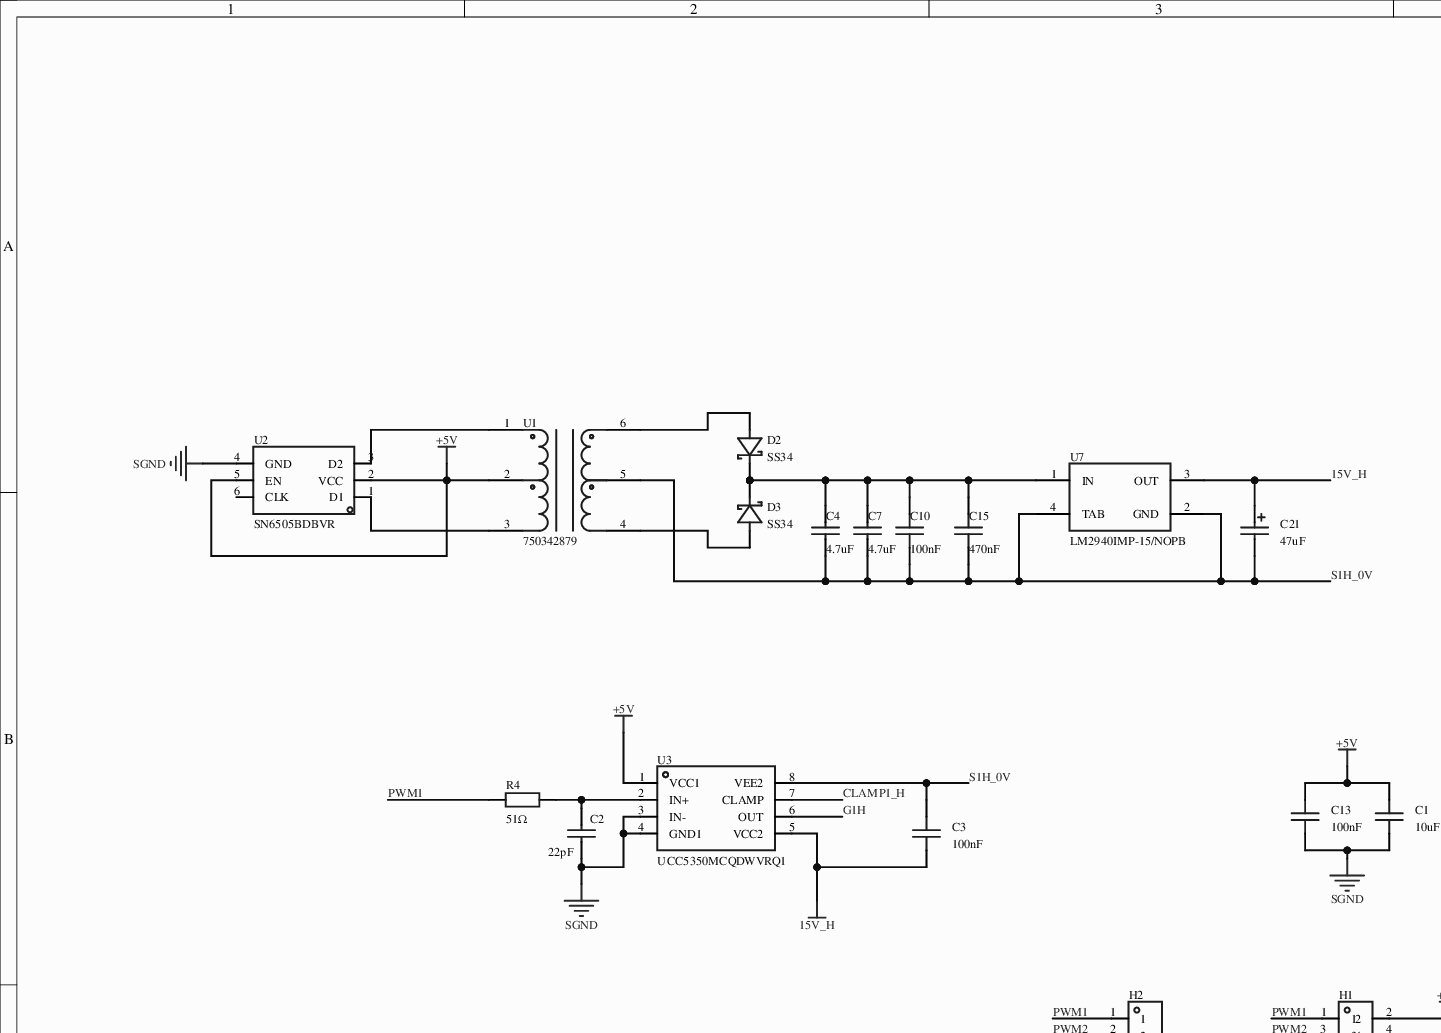
[diagram p0: MISC51425-3.schdoc, top left]
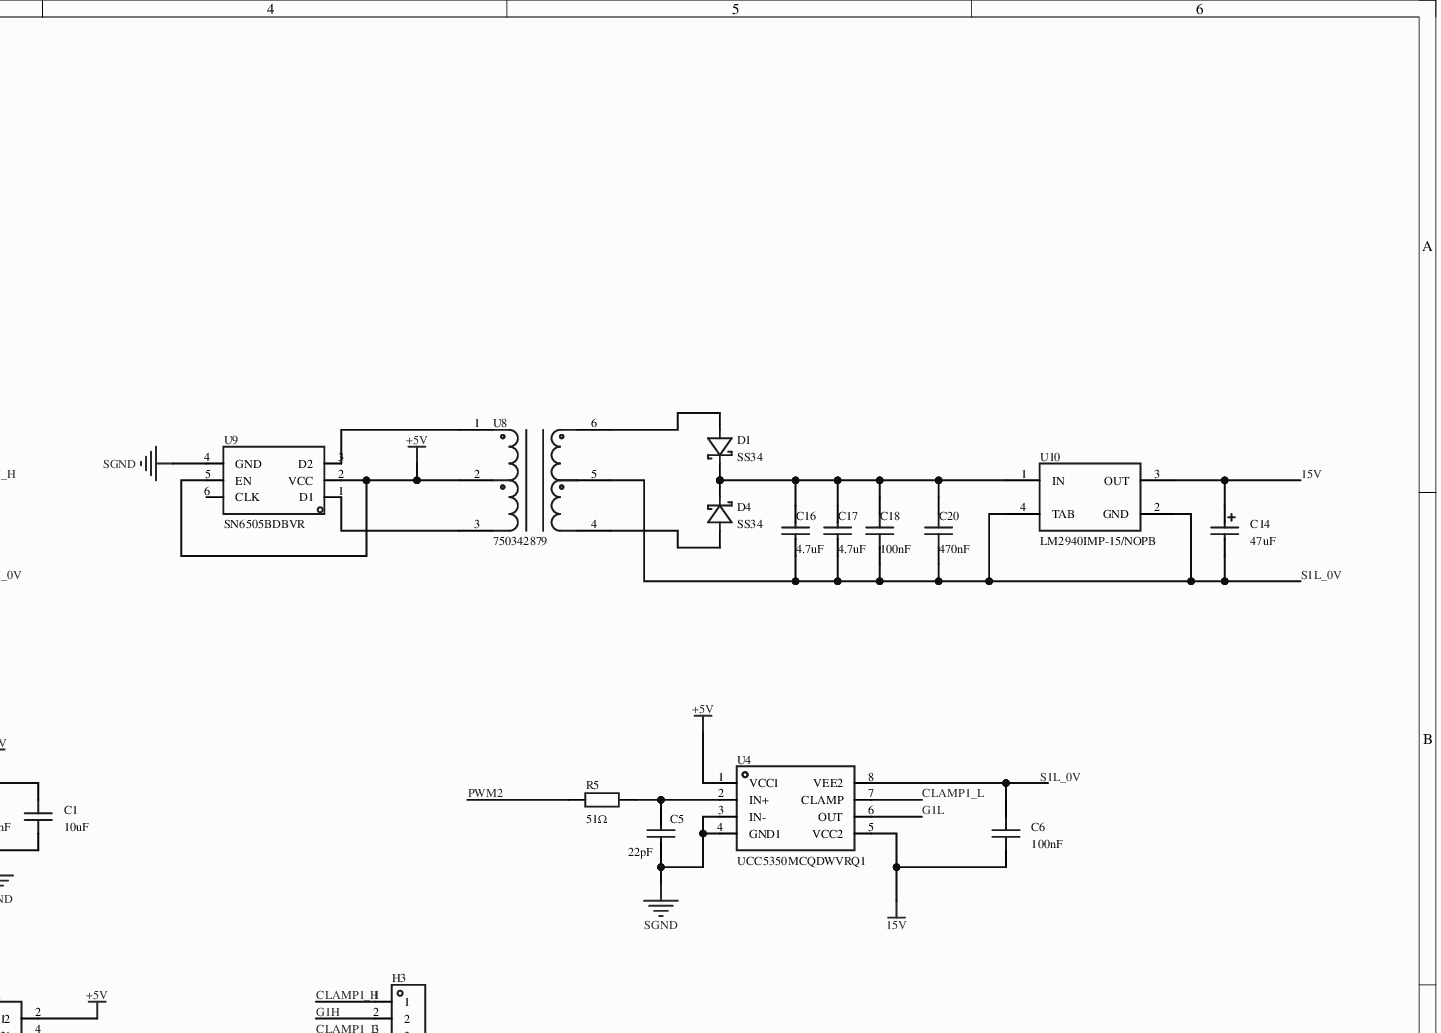
[diagram p1: MISC51425-3.schdoc, top right]
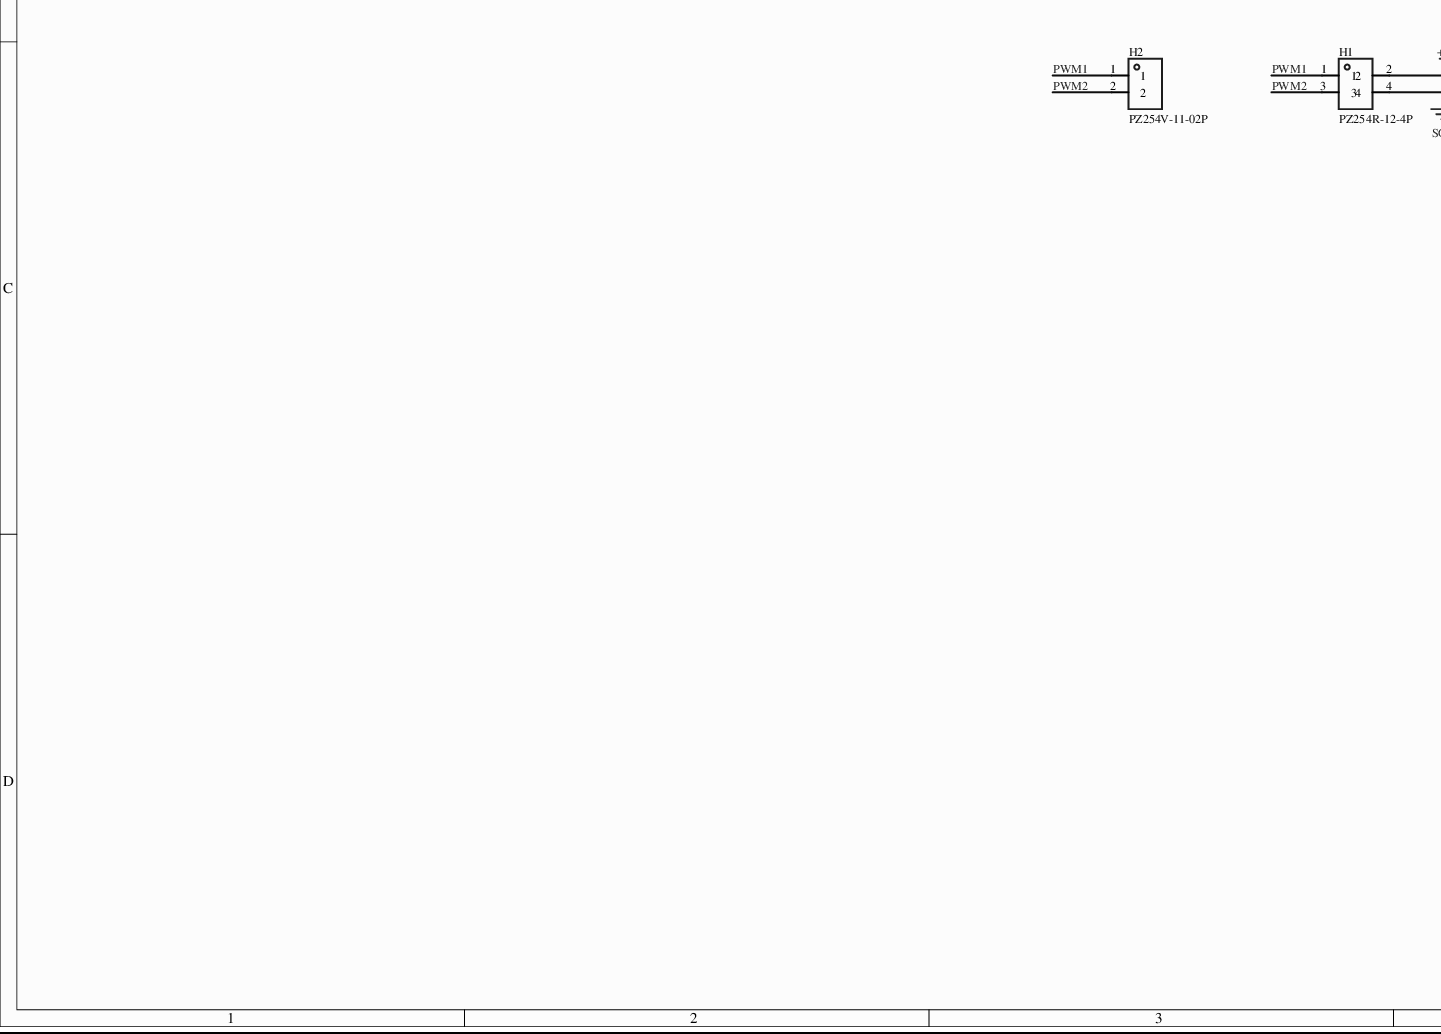
[diagram p2: MISC51425-3.schdoc, bottom left]
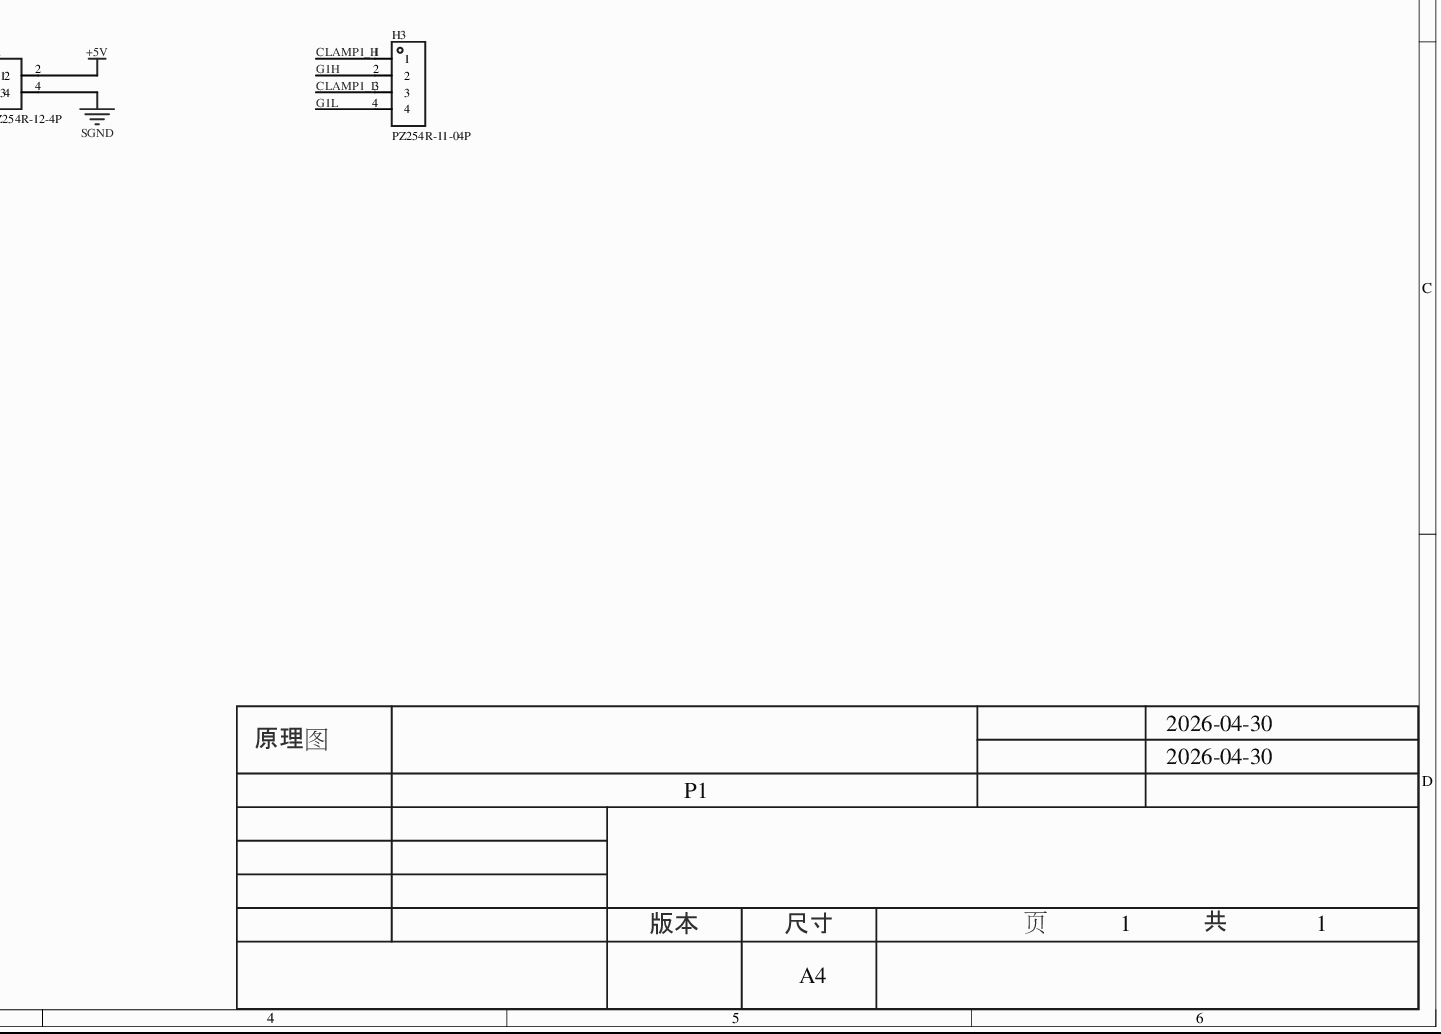
[diagram p3: MISC51425-3.schdoc, bottom right]
# Altium project MISC51425-2.PrjPcb
1 sheet, 33 parts. Net scope: global (net labels, ports and power ports of the same name join across sheets).
Board file: MISC51425.pcbdoc

## Sheet MISC51425-3.schdoc
size 420 x 297 mm; Version: V1.0; @Project Name: MISC51425; @Page Count: 1; @Update Date: 2026-04-30; @Create Date: 2026-04-30; @Schematic Name: MISC51425; @Page No: 1; @Board Name: MISC51425; @Update Time: 15:18:57; @Create Time: 15:18:57

### Parts
C1  10uF  [C0603]
C2  22pF  [C0402]
C3  100nF  [C0603]
C4  4.7uF  [C0805]
C5  22pF  [C0402]
C6  100nF  [C0603]
C7  4.7uF  [C0805]
C10  100nF  [CAP-SMD_L2.0-W1.25]
C13  100nF  [C0603]
C14  47uF  [CAP-SMD_L7.3-W4.3-FD]
C15  470nF  [C0603]
C16  4.7uF  [C0805]
C17  4.7uF  [C0805]
C18  100nF  [CAP-SMD_L2.0-W1.25]
C20  470nF  [C0603]
C21  47uF  [CAP-SMD_L7.3-W4.3-FD]
D1  SS34  [SMA_L4.3-W2.6-LS5.0-FD]
D2  SS34  [SMA_L4.3-W2.6-LS5.0-FD]
D3  SS34  [SMA_L4.3-W2.6-LS5.0-FD]
D4  SS34  [SMA_L4.3-W2.6-LS5.0-FD]
H1  PZ254R-12-4P  [HDR-TH_4P-P2.54-H-M-R2-C2-S2.54]
H2  PZ254V-11-02P  [HDR-TH_2P-P2.54-V-M]
H3  PZ254R-11-04P  [HDR-TH_4P-P2.54-H-M-W10.4]
R4  51Ω  [R0603]
R5  51Ω  [R0603]
U1  750342879  [XFMR-SMD_6P-L9.1-W8.0-P3.05-LS13.0-TL]
U2  SN6505BDBVR  [SOT-23-6_L2.9-W1.6-P0.95-LS2.8-BR]
U3  UCC5350MCQDWVRQ1  [SOIC-8_L7.5-W5.9-P1.27-LS11.5-BL]
U4  UCC5350MCQDWVRQ1  [SOIC-8_L7.5-W5.9-P1.27-LS11.5-BL]
U7  LM2940IMP-15/NOPB  [SOT-223-3_L6.5-W3.4-P2.30-LS7.0-BR]
U8  750342879  [XFMR-SMD_6P-L9.1-W8.0-P3.05-LS13.0-TL]
U9  SN6505BDBVR  [SOT-23-6_L2.9-W1.6-P0.95-LS2.8-BR]
U10  LM2940IMP-15/NOPB  [SOT-223-3_L6.5-W3.4-P2.30-LS7.0-BR]

### Nets
15V: C6.2 C14.1 U4.5(VCC2) U10.3(OUT)
15V_H: C3.2 C21.1 U3.5(VCC2) U7.3(OUT)
+5V: C1.1 C13.1 H1.2 U1.2 U2.2(VCC) U2.5(EN) U3.1(VCC1) U4.1(VCC1) U8.2 U9.2(VCC) U9.5(EN)
SGND: C1.2 C2.1 C5.1 C13.2 H1.4 U2.4(GND) U3.3(IN-) U3.4(GND1) U4.3(IN-) U4.4(GND1) U9.4(GND)
CLAMP1_H: H3.1 U3.7(CLAMP)
CLAMP1_L: H3.3 U4.7(CLAMP)
G1H: H3.2 U3.6(OUT)
G1L: H3.4 U4.6(OUT)
PWM1: H1.1 H2.1 R4.1
PWM2: H1.3 H2.2 R5.1
S1H_0V: C3.1 C4.1 C7.1 C10.1 C15.1 C21.2 U1.5 U3.8(VEE2) U7.2(GND) U7.4(TAB)
S1L_0V: C6.1 C14.2 C16.1 C17.1 C18.1 C20.1 U4.8(VEE2) U8.5 U10.2(GND) U10.4(TAB)
NetC2_2: C2.2 R4.2 U3.2(IN+)
NetC4_2: C4.2 C7.2 C10.2 C15.2 D2.2(K) D3.2(K) U7.1(IN)
NetC5_2: C5.2 R5.2 U4.2(IN+)
NetC16_2: C16.2 C17.2 C18.2 C20.2 D1.2(K) D4.2(K) U10.1(IN)
NetD1_1: D1.1(A) U8.6
NetD2_1: D2.1(A) U1.6
NetD3_1: D3.1(A) U1.4
NetD4_1: D4.1(A) U8.4
NetU1_1: U1.1 U2.3(D2)
NetU1_3: U1.3 U2.1(D1)
NetU8_1: U8.1 U9.3(D2)
NetU8_3: U8.3 U9.1(D1)

Not connected (* = marked no-connect by the designer): U2 6(CLK)*; U9 6(CLK)*

### Notes on the sheet
- 2026-04-30
- 原理图
- P1
- 版本
- 尺寸
- A4
- 页
- 1
- 共

### Library data of the parts
C1 = GRM188R61E106KA73D: 容值:10uF;精度:±10%;额定电压:25V;温度系数:X5R;; Manufacturer: muRata(村田); 3D Model: ac125912035d415993ca9572d50418b10819f05c4eef4c71ace90d822a990e87; 3D Model Transform: 62.992,31.496,0,0,0,0,0,0,0; Tolerance: ±10%; Voltage Rating: 25V; Temperature Coefficient: X5R; AddInBom: yes; ModelName: C0603_L1.6-W0.8-H0.8; Device: GRM188R61E106KA73D; Symbol: GRM188R61E106KA73D; LCSC Part Name: 10uF ±10% 25V; Supplier Part: C344022; Manufacturer Part: GRM188R61E106KA73D; Supplier Footprint: 0603; JLCPCB Part Class: Extended Part; Datasheet: https://item.szlcsc.com/datasheet/GRM188R61E106KA73D/320824.html; Supplier: LCSC; Value: 10uF; FootprintName: C0603; ConvertToPcb: yes
C2 C5 = 0402CG220J500NT: 容值:22pF;精度:±5%;额定电压:50V;温度系数:C0G;; Manufacturer: FH(风华); 3D Model: 36a51122f27c49738f86b3bfa98863e00819f05c4eef4c71ace90d822a990e87; 3D Model Transform: 39.37,19.685,0,0,0,0,0,0,0; Tolerance: ±5%; Voltage Rating: 50V; Temperature Coefficient: C0G; AddInBom: yes; ModelName: C0402_L1.0-W0.5-H0.5; Device: 0402CG220J500NT; Symbol: 0402CG220J500NT; LCSC Part Name: 22pF ±5% 50V; Supplier Part: C1555; Manufacturer Part: 0402CG220J500NT; Supplier Footprint: 0402; JLCPCB Part Class: Basic Part; Datasheet: https://item.szlcsc.com/datasheet/0402CG220J500NT/1907.html; Supplier: LCSC; Value: 22pF; FootprintName: C0402; ConvertToPcb: yes
C3 C6 C13 = CGA0603X7R104K500JT: 容值:100nF;精度:±10%;额定电压:50V;温度系数:X7R;; Manufacturer: HRE(芯声); 3D Model: ac125912035d415993ca9572d50418b10819f05c4eef4c71ace90d822a990e87; 3D Model Transform: 62.992,31.496,0,0,0,0,0,0,0; Tolerance: ±10%; Voltage Rating: 50V; Temperature Coefficient: X7R; AddInBom: yes; ModelName: C0603_L1.6-W0.8-H0.8; Device: CGA0603X7R104K500JT; Symbol: CGA0603X7R104K500JT; LCSC Part Name: 100nF ±10% 50V; Supplier Part: C6119867; Manufacturer Part: CGA0603X7R104K500JT; Supplier Footprint: 0603; JLCPCB Part Class: Extended Part; Datasheet: https://item.szlcsc.com/datasheet/CGA0603X7R104K500JT/7062573.html; Supplier: LCSC; Value: 100nF; FootprintName: C0603; ConvertToPcb: yes
C4 C7 C16 C17 = CL21A475KBQNNNE: 容值:4.7uF;精度:±10%;额定电压:50V;温度系数:X5R;; Manufacturer: SAMSUNG(三星); 3D Model: 1ba041120af144c991958decab20d2410819f05c4eef4c71ace90d822a990e87; 3D Model Transform: 78.74,51.181,0,0,0,0,0,0.0005,0; Tolerance: ±10%; Voltage Rating: 50V; Temperature Coefficient: X5R; AddInBom: yes; ModelName: C0805_L2.0-W1.3-H1.3; Device: CL21A475KBQNNNE; Symbol: CL21A475KBQNNNE; LCSC Part Name: 4.7uF ±10% 50V; Supplier Part: C98192; Manufacturer Part: CL21A475KBQNNNE; Supplier Footprint: 0805; JLCPCB Part Class: Extended Part; Datasheet: https://item.szlcsc.com/datasheet/CL21A475KBQNNNE/99401.html; Supplier: LCSC; Value: 4.7uF; FootprintName: C0805; ConvertToPcb: yes
C10 C18 = FCC0805B104K500DT: 容值:100nF;精度:±10%;额定电压:50V;温度系数:X7R;; Manufacturer: FOJAN(富捷); 3D Model: dce19e309e9b4209af79576cb8c62f2f0819f05c4eef4c71ace90d822a990e87; 3D Model Transform: 78.74,49.2125,0,0,0,0,0,0,0; Tolerance: ±10%; Voltage Rating: 50V; Temperature Coefficient: X7R; AddInBom: yes; ModelName: CAP-SMD_L2.0-W1.3-H1.3; Device: FCC0805B104K500DT; Symbol: FCC0805B104K500DT; LCSC Part Name: 100nF ±10% 50V; Supplier Part: C5137467; Manufacturer Part: FCC0805B104K500DT; Supplier Footprint: 0805; JLCPCB Part Class: Extended Part; Datasheet: https://item.szlcsc.com/datasheet/FCC0805B104K500DT/5746969.html; Supplier: LCSC; Value: 100nF; FootprintName: CAP-SMD_L2.0-W1.25; ConvertToPcb: yes
C14 C21 = T491X476K035AT: 容值:47uF;精度:±10%;额定电压:35V;等效串联电阻(ESR):600mΩ@100kHz;; Manufacturer: KEMET(基美); 3D Model: a7253e4667014c2b8171994ff34e6c410819f05c4eef4c71ace90d822a990e87; 3D Model Transform: 287.402,169.291,0,0,0,0,-0.1,0,0; Tolerance: ±10%; Voltage Rating: 35V; AddInBom: yes; ModelName: CASE-E_L7.3-W4.3-H4.1; Device: T491X476K035AT; Symbol: T491X476K035AT; LCSC Part Name: 47uF ±10% 35V; Supplier Part: C87110; Manufacturer Part: T491X476K035AT; Supplier Footprint: CASE-X-7343-43(mm); JLCPCB Part Class: Extended Part; Datasheet: https://item.szlcsc.com/datasheet/T491X476K035AT/88288.html; Supplier: LCSC; Value: 47uF; Equivalent Series Resistance(ESR): 600mΩ@100kHz; Operating Temperature: -55℃~+125℃; FootprintName: CAP-SMD_L7.3-W4.3-FD; ConvertToPcb: yes
C15 C20 = CC0603KRX7R9BB474: 容值:470nF;精度:±10%;额定电压:50V;温度系数:X7R;; Manufacturer: YAGEO(国巨); 3D Model: ac125912035d415993ca9572d50418b10819f05c4eef4c71ace90d822a990e87; 3D Model Transform: 62.992,31.496,0,0,0,0,0,0,0; Tolerance: ±10%; Voltage Rating: 50V; Temperature Coefficient: X7R; AddInBom: yes; ModelName: C0603_L1.6-W0.8-H0.8; Device: CC0603KRX7R9BB474; Symbol: CC0603KRX7R9BB474; LCSC Part Name: 470nF ±10% 50V; Supplier Part: C513577; Manufacturer Part: CC0603KRX7R9BB474; Supplier Footprint: 0603; JLCPCB Part Class: Extended Part; Datasheet: https://item.szlcsc.com/datasheet/CC0603KRX7R9BB474/528404.html; Supplier: LCSC; Value: 470nF; FootprintName: C0603; ConvertToPcb: yes
D1-D4 = SS34_C7420365: 二极管配置:独立式;正向压降(Vf):550mV@3A;直流反向耐压(Vr):40V;整流电流:3A;; Manufacturer: R+O(宏嘉诚); 3D Model: 7e24bebe6cd74171ae8c9de6fc5b78aa0819f05c4eef4c71ace90d822a990e87; 3D Model Transform: 198.4248,103.5431,0,180,0,0,-0.001,0,0; Diode Configuration: 独立式; Voltage - DC Reverse(Vr): 40V; Current - Rectified: 3A; Reverse Leakage Current (Ir): 200uA@40V; AddInBom: yes; Device: SS34_C7420365; Symbol: SS34_C7420365; LCSC Part Name: 电压:40V 电流:3A; Supplier Part: C7420365; Manufacturer Part: SS34; Supplier Footprint: SMA(DO-214AC); JLCPCB Part Class: Extended Part; Datasheet: https://item.szlcsc.com/datasheet/SS34/8397187.html; Supplier: LCSC; Voltage - Forward(Vf@If): 550mV@3A; FootprintName: SMA_L4.3-W2.6-LS5.0-FD; ConvertToPcb: yes; ModelName: SMA_L4.3-W2.6-LS5.0-FD
H1 = PZ254R-12-4P: 插针结构:2x2P;间距:2.54mm;行距:2.54mm;圆针/方针:方针;安装方式:弯插;排数:双排;总PIN位数:4P;额定电流:-;额定电压:-;配合针长度:6mm;塑高:2.5mm;触头材质:黄铜;触头镀层:-;工作温度:-40℃~+105℃;颜色:黑色;; Manufacturer: XFCN(兴飞); 3D Model: 0bf87f84c3ca4f928641a0c742925de30819f05c4eef4c71ace90d822a990e87; 3D Model Transform: 200,507.873,0,0,0,0,0,-190.945,-118.11; Pin Structure: 2x2P; Pitch: 2.54mm; Circluar Pins/Square Pins: 方针; AddInBom: yes; ModelName: HDR-TH_4P-P2.54-M-WI-2X2P; Device: PZ254R-12-4P; Symbol: PZ254R-12-4P; LCSC Part Name: 2x2P 间距:2.54mm 方针 弯插; Supplier Part: C492430; Manufacturer Part: PZ254R-12-4P; Supplier Footprint: 弯插,P=2.54mm; JLCPCB Part Class: Extended Part; Datasheet: https://atta.szlcsc.com/upload/public/pdf/source/20200309/C492430_40F61060098E2A512B5822C8CF53ABE1.pdf; Supplier: LCSC; Row Spacing: 2.54mm; Mounting Type: 弯插; Number of Rows: 双排; Number of Pins: 4P; Current Rating: -; Voltage Rating (Max): -; Length of Mating Pin: 6mm; Insulation Height: 2.5mm; Contact Material: 黄铜; Contact Plating: -; Operating Temperature: -40℃~+105℃; Color: 黑色; FootprintName: HDR-TH_4P-P2.54-H-M-R2-C2-S2.54; ConvertToPcb: yes
H2 = PZ254V-11-02P: 插针结构:1x2P;间距:2.54mm;行距:-;圆针/方针:方针;安装方式:直插;排数:单排;总PIN位数:2P;额定电流:3A;额定电压:250V;配合针长度:6mm;塑高:2.5mm;端接针长度:3mm;触头材质:黄铜;触头镀层:-;工作温度:-40℃~+105℃;颜色:黑色;; Manufacturer: XFCN(兴飞); 3D Model: e35305ec3aa84b66b849f914b715e73f0819f05c4eef4c71ace90d822a990e87; 3D Model Transform: 200,100,0,0,0,0,0,0,-118.11; Pin Structure: 1x2P; Pitch: 2.54mm; Circluar Pins/Square Pins: 方针; Current Rating: 3A; Voltage Rating (Max): 250V; AddInBom: yes; ModelName: HDR2.54-M-LI-1X2P; Device: PZ254V-11-02P; Symbol: PZ254V-11-02P; LCSC Part Name: 1x2P 间距:2.54mm 方针 直插; Supplier Part: C492401; Manufacturer Part: PZ254V-11-02P; Supplier Footprint: 插件,P=2.54mm; JLCPCB Part Class: Extended Part; Datasheet: https://item.szlcsc.com/datasheet/PZ254V-11-02P/502957.html; Supplier: LCSC; Row Spacing: -; Mounting Type: 直插; Number of Rows: 单排; Number of Pins: 2P; Length of Mating Pin: 6mm; Insulation Height: 2.5mm; Length of End Connection Pin: 3mm; Contact Material: 黄铜; Contact Plating: -; Operating Temperature: -40℃~+105℃; Color: 黑色; FootprintName: HDR-TH_2P-P2.54-V-M; ConvertToPcb: yes
H3 = PZ254R-11-04P: 插针结构:1x4P;间距:2.54mm;行距:-;圆针/方针:方针;安装方式:弯插;排数:单排;总PIN位数:4P;额定电流:3A;额定电压:250V;配合针长度:6mm;塑高:2.5mm;端接针长度:-;触头材质:黄铜;触头镀层:-;工作温度:-40℃~+105℃;颜色:黑色;; Manufacturer: XFCN(兴飞); 3D Model: d6c429cf28314298a2074cefd68172f00819f05c4eef4c71ace90d822a990e87; 3D Model Transform: 399.999,417.322,0,180,0,0,0,-196.85,-118.11; Pin Structure: 1x4P; Pitch: 2.54mm; Circluar Pins/Square Pins: 方针; Current Rating: 3A; Voltage Rating (Max): 250V; AddInBom: yes; ModelName: HDR-TH_4P-P2.54-M-WI-1X4P; Device: PZ254R-11-04P; Symbol: PZ254R-11-04P; LCSC Part Name: 1x4P 间距:2.54mm 方针 弯插; Supplier Part: C492412; Manufacturer Part: PZ254R-11-04P; Supplier Footprint: 弯插,P=2.54mm; JLCPCB Part Class: Extended Part; Datasheet: https://item.szlcsc.com/datasheet/PZ254R-11-04P/502968.html; Supplier: LCSC; Row Spacing: -; Mounting Type: 弯插; Number of Rows: 单排; Number of Pins: 4P; Length of Mating Pin: 6mm; Insulation Height: 2.5mm; Length of End Connection Pin: -; Contact Material: 黄铜; Contact Plating: -; Operating Temperature: -40℃~+105℃; Color: 黑色; FootprintName: HDR-TH_4P-P2.54-H-M-W10.4; ConvertToPcb: yes
R4 R5 = 0603WAF510JT5E: 电阻类型:厚膜电阻;阻值:51Ω;精度:±1%;功率:100mW;工作电压:75V;温度系数:±100ppm/℃;; Manufacturer: UNI-ROYAL(厚声); 3D Model: fc143cca1e79419f9cd78b61e9279f080819f05c4eef4c71ace90d822a990e87; 3D Model Transform: 31.8897,63.7794,0,90,0,0,0,0,0; Tolerance: ±1%; Power(Watts): 100mW; Voltage-Supply(Max): 75V; AddInBom: yes; Device: 0603WAF510JT5E; Symbol: 0603WAF510JT5E; LCSC Part Name: 51Ω ±1% 100mW 厚膜电阻; Supplier Part: C23197; Manufacturer Part: 0603WAF510JT5E; Supplier Footprint: 0603; JLCPCB Part Class: Basic Part; Datasheet: https://item.szlcsc.com/datasheet/0603WAF510JT5E/23924.html; Supplier: LCSC; Type: 厚膜电阻; Value: 51Ω; Temperature Coefficient: ±100ppm/℃; Operating Temperature: -55℃~+155℃; FootprintName: R0603; ConvertToPcb: yes; ModelName: R0603
U1 U8 = 750342879: Manufacturer: Wurth(伍尔特); 3D Model: d40274c61c8d473899a1eceb1be707720819f05c4eef4c71ace90d822a990e87; 3D Model Transform: 509.842,359.8418,0,0,0,0,0,0,0; AddInBom: yes; Device: 750342879; Symbol: 750342879; LCSC Part Name: 750342879; Supplier Part: C5343012; Manufacturer Part: 750342879; Supplier Footprint: SMD-6P,9.1x8mm; JLCPCB Part Class: Extended Part; Datasheet: https://www.we-online.com/components/products/datasheet/750342879.pdf; Supplier: LCSC; FootprintName: XFMR-SMD_6P-L9.1-W8.0-P3.05-LS13.0-TL; ConvertToPcb: yes; ModelName: XFMR-SMD_6P-L9.1-W8.0-P3.05-LS13.0-TL
U2 U9 = SN6505BDBVR: SN6505B 适用于隔离电源的低噪声、1A、420kHz 变压器驱动器; Manufacturer: TI(德州仪器); Symbol: SN6505BDBVT; 3D Model: 18da8f6c14a34920b3e136b5c401a1190819f05c4eef4c71ace90d822a990e87; 3D Model Transform: 110.73671,114.173,0,180,0,0,0.001,-0.003,0; AddInBom: yes; ModelName: SOT-23-6_L2.9-W1.6-H1.5-LS2.8-P0.95; Device: SN6505BDBVR; LCSC Part Name: SN6505BDBVR; Supplier Part: C74518; Manufacturer Part: SN6505BDBVR; Supplier Footprint: SOT-23-6; JLCPCB Part Class: Extended Part; Datasheet: https://www.ti.com/cn/lit/gpn/sn6505b; Supplier: LCSC; FootprintName: SOT-23-6_L2.9-W1.6-P0.95-LS2.8-BR; ConvertToPcb: yes
U3 U4 = UCC5350MCQDWVRQ1: UCC5350-Q1 是一款单通道隔离式栅极驱动器，具有 5A 最小峰值拉电流和 5A 最小峰值灌电流，专为驱动 MOSFET、IGBT 和 SiC MOSFET 而设计。UCC5350-Q1 具有米勒钳位或分离输出选项。CLAMP 引脚除了可将晶体管栅极连接到输出端之外，还用于将栅极连接到内部 FET，以防止米勒电流造成假接通。借助分离输出选项，可以使用 OUTH 和 OUTL 引脚单独控制栅极电压的上升和下降时间。UCC5350-Q1 采用 4mm SOIC-8 (D) 或 8.5mm 宽体 SOIC; Manufacturer: TI(德州仪器); 3D Model: 0c2b0c5769684830a3d8e8d39172fb8a0819f05c4eef4c71ace90d822a990e87; 3D Model Transform: 452.755,230.315,0,90,0,0,0,0,0; AddInBom: yes; Device: UCC5350MCQDWVRQ1; Symbol: UCC5350MCQDWVRQ1; LCSC Part Name: 单通道隔离式栅极驱动器，适用于SiC/IGBT器件和汽车应用; Supplier Part: C2871469; Manufacturer Part: UCC5350MCQDWVRQ1; Supplier Footprint: SOIC-8; JLCPCB Part Class: Extended Part; Datasheet: https://www.ti.com/cn/lit/gpn/ucc5350-q1; Supplier: LCSC; FootprintName: SOIC-8_L7.5-W5.9-P1.27-LS11.5-BL; ConvertToPcb: yes; ModelName: SOIC-8_L7.5-W5.9-P1.27-LS11.5-BL
U7 U10 = LM2940IMP-15/NOPB: 输出类型:固定;工作电压:26V;输出电压:15V;输出电流:1A;电源纹波抑制比(PSRR):-;输出极性:正极;; Manufacturer: TI(德州仪器); 3D Model: 925194bf9823436183a3e0b978a8d0760819f05c4eef4c71ace90d822a990e87; 3D Model Transform: 279.89794,255.905,0,180,0,0,-3.9385,-0.0005,0; Output Type: 固定; Voltage - Supply: 26V; Output Voltage: 15V; Output Current: 1A; Voltage Dropout: 1V@(1A); Output Configuration: 正极; Number of Outputs: 1; AddInBom: yes; ModelName: SOT-223-4P_L6.5-W3.5-H1.6-LS7.0-P2.30; Device: LM2940IMP-15/NOPB; Symbol: LM2940IMP-15/NOPB; LCSC Part Name: 1A、26V、高 PSRR、低压降稳压器; Supplier Part: C81094; Manufacturer Part: LM2940IMP-15/NOPB; Supplier Footprint: SOT-223-3; JLCPCB Part Class: Extended Part; Datasheet: https://www.ti.com/cn/lit/gpn/lm2940c; Supplier: LCSC; Power Supply Rejection Ratio (PSRR): -; Features: 防静电保护；欠压锁定；过热保护；过压保护；过流保护；短路保护; FootprintName: SOT-223-3_L6.5-W3.4-P2.30-LS7.0-BR; ConvertToPcb: yes